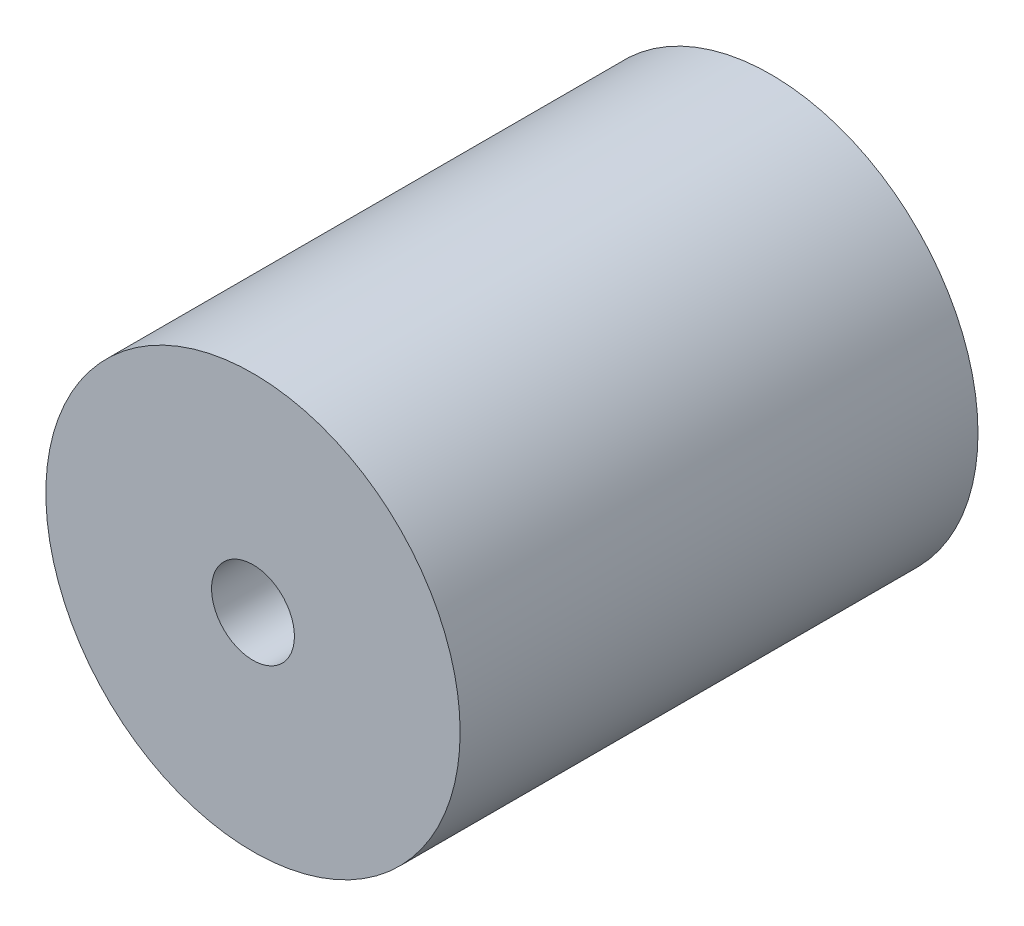
from build123d import *

# Parameters (mm, degrees)
SKETCH_1_R      = 20
SKETCH_1_R_2    = 4
EXTRUDE_1_DEPTH = 50


with BuildPart() as part:
    # 草图1 → 凸台-拉伸1 (new body)
    with BuildSketch(Plane.XY):
        Circle(SKETCH_1_R)
        Circle(SKETCH_1_R_2, mode=Mode.SUBTRACT)
    extrude(amount=EXTRUDE_1_DEPTH)


solid = part.part
